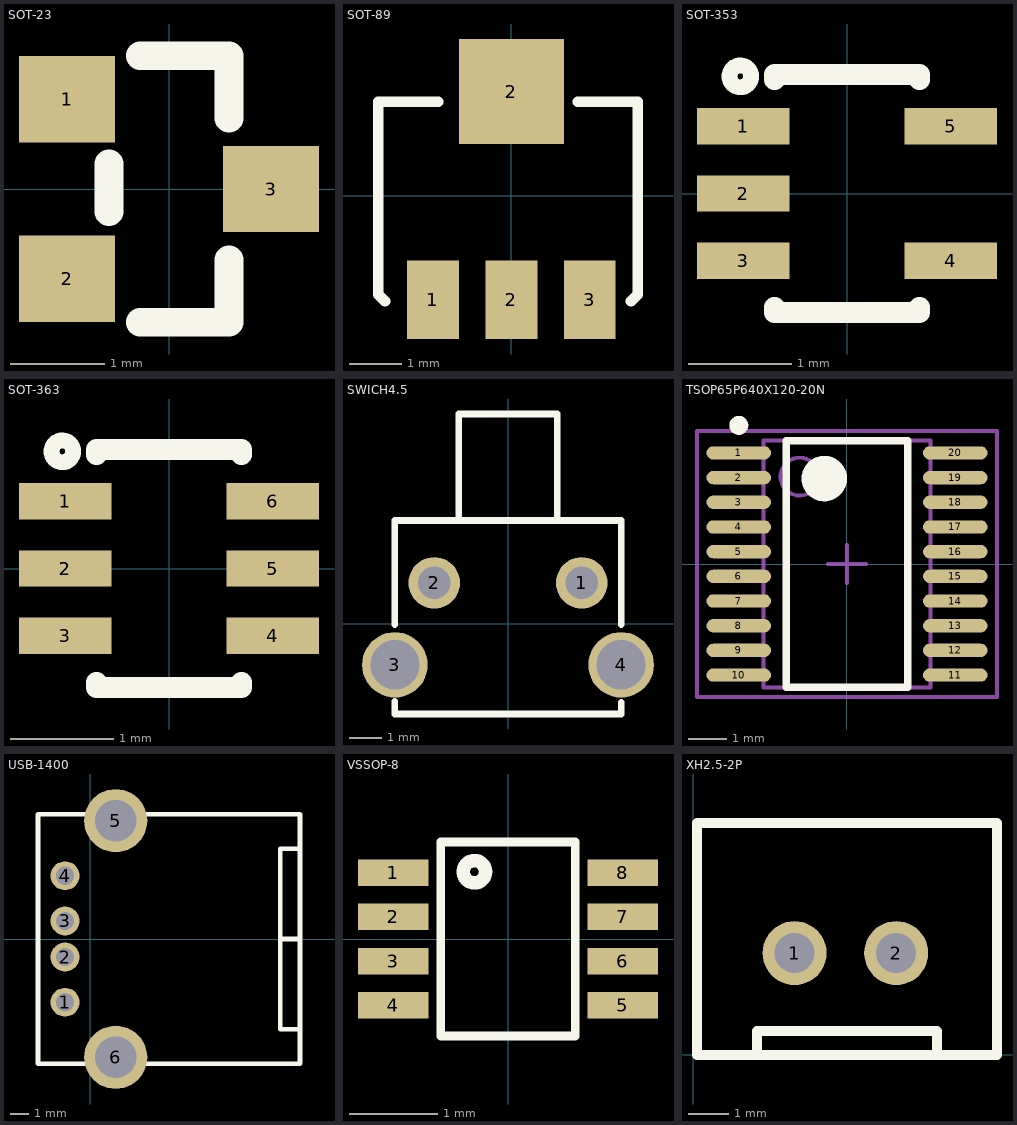
[diagram p0: the footprints below, top view; thin cyan lines are the x and y axes]
# Altium footprint library MISC82794-2.PcbLib: 41 footprints (part 3 of 3)
Each footprint in its own frame and in the unit in brackets; x right, y up, seen from the top. Pads: shape width x height; smd on the part's side, far side on the other; paste and mask are expansions set on the pad; w line width, h text height; cw(c..) or ccw(c..) is an arc to the next point about the centre after c.

## SOT-23 [mil]
height 374.02
pads (3):
  rect 40x36 smd: 1(-42.5,37.4) 2(-42.5,-37.4) 3(42.5,0)
Top Overlay:
  lines w12: -25,-9.5 -25,10.5 ; -12,-55.5 25,-55.5 25,-29.5 ; -12,55.5 25,55.5 25,29.5
3D body: height 39.37, standoff -0.79, extent -47,-56.98 50.48,57.98

## SOT-89 [mil]
height 47.24
pads (4):
  rect 39x59 smd: 1(-59,-78.3) 2(0,-78.3) 3(59,-78.3)
  rect 79x79 smd: 2(0,78.3)
Top Overlay:
  lines w8: -95,-79.3 -100,-74.3 -100,70.7 -55,70.7 ; 50,70.7 95,70.7 95,-74.3 90,-79.3

## SOT-353 [mm]
height 9.5
pads (5):
  rect 0.896x0.35 smd: 1(-1.002,0.65) 2(-1.002,0) 3(-1.002,-0.65) 4(1.002,-0.65) 5(1.002,0.65)
Top Overlay:
  circle w0.152: c-1.031,1.133 r0.105
  lines w0.2: -0.7,-1.1 -0.7,-1.15 0.7,-1.15 0.7,-1.1 ; -0.7,1.1 -0.7,1.15 0.7,1.15 0.7,1.1

## SOT-363 [mm]
height 1.016
pads (6):
  rect 0.896x0.35 smd: 1(-1.002,0.65) 2(-1.002,0) 3(-1.002,-0.65) 4(1.002,-0.65) 5(1.002,0) 6(1.002,0.65)
Top Overlay:
  circle w0.152: c-1.031,1.133 r0.105
  lines w0.2: -0.7,-1.1 -0.7,-1.15 0.7,-1.15 0.7,-1.1 ; -0.7,1.1 -0.7,1.15 0.7,1.15 0.7,1.1
3D body: height 1, standoff 0, extent -1.15,-1.041 1.15,1.059

## SWICH4.5 [mm] "6.6mm"
pads (4):
  round 1.575 hole 1: 1(2.25,1.25) 2(-2.25,1.25)
  round 2 hole 1.5: 3(-3.45,-1.25) 4(3.45,-1.25)
Top Overlay:
  lines w0.203: -3.45,-2.361 -3.45,-2.75 3.45,-2.75 3.45,-2.387 ; -3.45,-0.02 -3.45,3.15 3.454,3.15 3.454,-0.02 ; -1.5,3.15 -1.5,6.4 1.5,6.4 1.5,3.15

## TSOP65P640X120-20N [mm] "TSOP, 20-Leads, Body 6.5x4.4mm (max), Pitch 0.65"
height 1.2
pads (20):
  oval 1.7x0.35 smd: 1(-2.85,2.925) 2(-2.85,2.275) 3(-2.85,1.625) 4(-2.85,0.975) 5(-2.85,0.325) 6(-2.85,-0.325) 7(-2.85,-0.975) 8(-2.85,-1.625) 9(-2.85,-2.275) 10(-2.85,-2.925) 11(2.85,-2.925) 12(2.85,-2.275) 13(2.85,-1.625) 14(2.85,-0.975) 15(2.85,-0.325) 16(2.85,0.325) 17(2.85,0.975) 18(2.85,1.625) 19(2.85,2.275) 20(2.85,2.925)
Top Overlay:
  circle w0.6: c-0.6,2.25 r0.3
  circle w0.25: c-2.85,3.65 r0.125
  lines w0.2: -1.6,-3.25 1.6,-3.25 1.6,3.25 -1.6,3.25 -1.6,-3.25
Mechanical 13:
  circle w0.1: c-1.25,2.3 r0.5
  lines w0.1: -2.2,-3.25 2.2,-3.25 2.2,3.25 -2.2,3.25 -2.2,-3.25
Mechanical 15:
  lines w0.1: -0.5,0 0.5,0 ; 0,-0.5 0,0.5 ; -3.95,-3.5 3.95,-3.5 3.95,3.5 -3.95,3.5 -3.95,-3.5
3D body: height 1.2, standoff 0.09, extent -2.2,-3.25 2.2,3.25

## USB-1400 [mm] "5.5mm"
pads (6):
  round 1.6 hole 1: 1(-1.4,-3.5) 2(-1.4,-1) 3(-1.4,1) 4(-1.4,3.5)
  round 3.5 hole 2.3: 5(1.4,6.55) 6(1.4,-6.55)
Top Overlay:
  lines w0.254: 10.5,0 11.6,0 ; 11.5,-5 10.5,-5 10.5,5 11.6,5 ; -2.9,-6.9 11.6,-6.9 11.6,6.9 -2.9,6.9 -2.9,-6.9

## VSSOP-8 [mm]
height 3.98
pads (8):
  rect 0.8x0.3 smd: 1(-1.3,0.75) 2(-1.3,0.25) 3(-1.3,-0.25) 4(-1.3,-0.75) 5(1.3,-0.75) 6(1.3,-0.25) 7(1.3,0.25) 8(1.3,0.75)
Top Overlay:
  circle w0.152: c-0.381,0.762 r0.127
  lines w0.1: -0.762,-1.1 0.762,-1.1 0.762,1.1 -0.762,1.1 -0.762,-1.1

## XH2.5-2P [mm]
pads (2):
  round 1.6 hole 1: 1(2.54,2.54) 2(5.08,2.54)
Top Overlay:
  lines w0.254: 1.599,-0.007 1.599,0.593 6.1,0.593 6.1,0 ; 0.099,-0.007 7.6,-0.007 7.6,5.793 0.099,5.793 0.099,-0.007